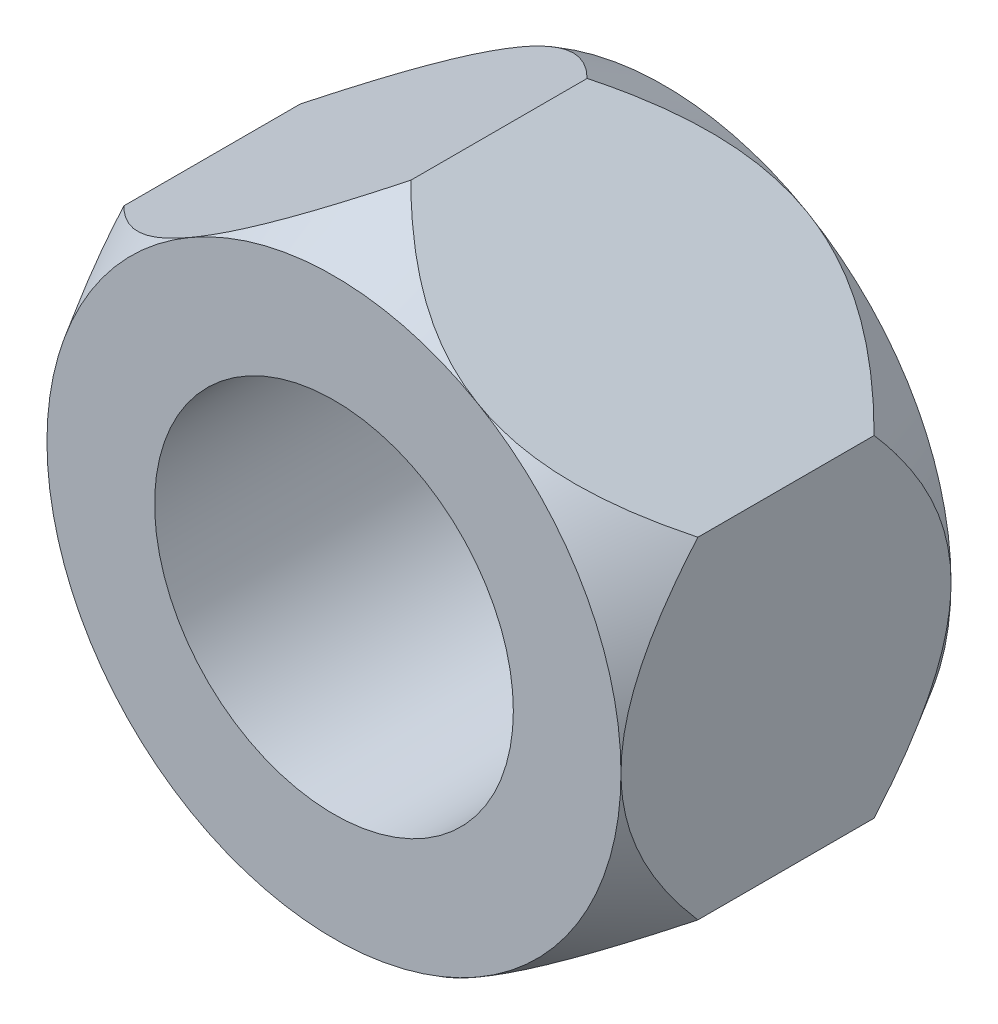
SolidWorks part; units mm, degrees
ref_plane "Front Plane" through (0, 0, 0) normal (0, 0, 1) x (1, 0, 0)
ref_plane "Top Plane" through (0, 0, 0) normal (0, 1, 0) x (1, 0, 0)
ref_plane "Right Plane" through (0, 0, 0) normal (1, 0, 0) x (0, 0, -1)
sketch "Sketch1" plane through (0, 0, 0) normal (0, 0, 1) x (1, 0, 0)
  line L1 (0, 23.094) -> (-20, 11.547)
  line L2 (-20, 11.547) -> (-20, -11.547)
  line L3 (-20, -11.547) -> (0, -23.094)
  line L4 (0, -23.094) -> (20, -11.547)
  line L5 (20, -11.547) -> (20, 11.547)
  line L6 (20, 11.547) -> (0, 23.094)
  circle A0 centre (0, 0) radius 20 construction
  dimension "D1" = 40
extrude "Boss-Extrude1" add sketch "Sketch1" along normal mid plane 23
sketch "Sketch2" plane through (0, 0, 11.5) normal (0, 0, 1) x (1, 0, 0)
  line L0 (20, 11.547) -> (0, 23.094) construction
  circle A0 centre (0, 0) radius 20
extrude "Cut-Extrude1" cut sketch "Sketch2" against normal blind 18 draft 30 flip side to cut
mirror "Mirror1" about plane through (0, 0, 0) normal (0, 0, 1) of "Cut-Extrude1"
sketch "Sketch3" plane through (0, 0, 11.5) normal (0, 0, 1) x (1, 0, 0)
  circle A0 centre (0, 0) radius 12.5
  dimension "D1" = 25
extrude "Cut-Extrude2" cut sketch "Sketch3" against normal blind 18
sketch "Sketch4" plane through (0, 0, -6.5) normal (0, 0, 1) x (1, 0, 0)
  circle A0 centre (0, 0) radius 6
  dimension "D1" = 12
extrude "Cut-Extrude3" cut sketch "Sketch4" against normal blind 18
